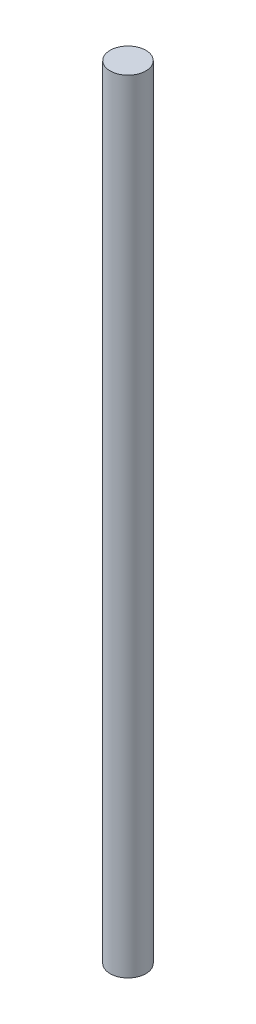
from build123d import *

# Parameters (mm, degrees)
SKETCH1_R           = 0.8
BOSS_EXTRUDE1_DEPTH = 35


with BuildPart() as part:
    # Sketch1 → Boss-Extrude1 (new body)
    with BuildSketch(Plane(origin=(0, 0, 0), x_dir=(1, 0, 0), z_dir=(0, 1, 0))):
        with Locations(Location((0, 0, 0), (0, 0, 270))):
            Circle(SKETCH1_R)
    extrude(amount=BOSS_EXTRUDE1_DEPTH)


solid = part.part
